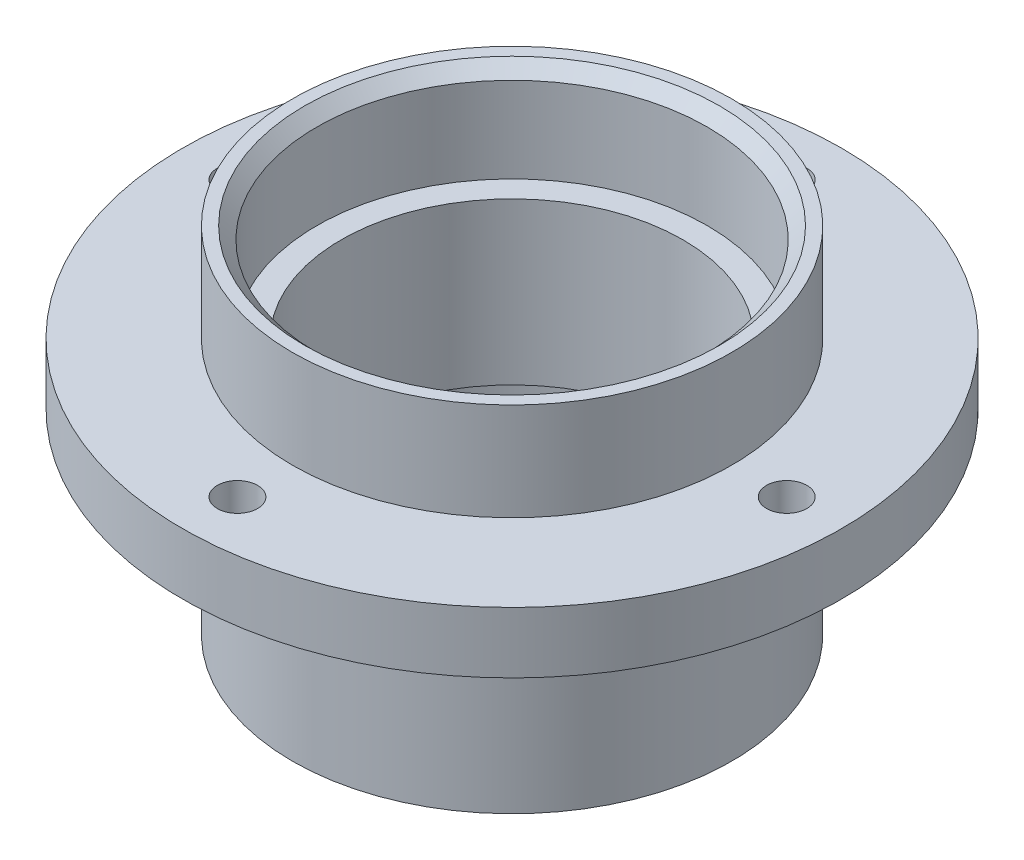
from build123d import *

# Parameters (mm, degrees)
SKETCH1_R             = 18
BOSS_EXTRUDE1_DEPTH   = 8
CUT_EXTRUDE1_REACH    = 28.683
SKETCH2_R             = 16
SKETCH3_R             = 27
BOSS_EXTRUDE2_DEPTH   = 5
BOSS_EXTRUDE3_START   = 16
SKETCH4_R             = 18
BOSS_EXTRUDE3_DEPTH   = 16
SKETCH5_R             = 16
CUT_EXTRUDE2_DEPTH    = 7.8
SKETCH6_R             = 14
CUT_EXTRUDE3_DEPTH    = 44.577517139
M4_TAPPED_HOLE1_D     = 3.3
M4_TAPPED_HOLE1_DEPTH = 11.5
M4_TAPPED_HOLE1_TIP   = 0.991420021
CHAMFER1_SIZE         = 1


with BuildPart() as part:
    # Sketch1 → Boss-Extrude1 (new body)
    with BuildSketch(Plane(origin=(0, 0, 0), x_dir=(1, 0, 0), z_dir=(0, 1, 0))):
        with Locations(Location((0, 0, 0), (0, 0, 270))):
            Circle(SKETCH1_R)
    extrude(amount=BOSS_EXTRUDE1_DEPTH)

    # Sketch2 → Cut-Extrude1 (cut, up to next)
    with BuildSketch(Plane.XZ, mode=Mode.PRIVATE) as cut_extrude1_sk1:
        with Locations(Location((0, 0, 0), (0, 0, 270))):
            Circle(SKETCH2_R)
    cut_extrude1_tool1 = extrude(cut_extrude1_sk1.sketch, amount=-CUT_EXTRUDE1_REACH, mode=Mode.PRIVATE) & part.part
    add(cut_extrude1_tool1.solids().sort_by_distance((0, 0, 0))[0], mode=Mode.SUBTRACT)

    # Sketch3 → Boss-Extrude2 (add)
    with BuildSketch(Plane.XZ):
        with Locations(Location((0, 0, 0), (0, 0, 270))):
            Circle(SKETCH3_R)
    extrude(amount=BOSS_EXTRUDE2_DEPTH)

    # Sketch4 → Boss-Extrude3 (add)
    with BuildSketch(Plane.XZ.offset(5).offset(BOSS_EXTRUDE3_START)):
        with Locations(Location((0, 0, 0), (0, 0, 270))):
            Circle(SKETCH4_R)
    extrude(amount=-BOSS_EXTRUDE3_DEPTH)

    # Sketch5 → Cut-Extrude2 (cut)
    with BuildSketch(Plane.XZ.offset(21)):
        with Locations(Location((0, 0, 0), (0, 0, 270))):
            Circle(SKETCH5_R)
    extrude(amount=-CUT_EXTRUDE2_DEPTH, mode=Mode.SUBTRACT)

    # Sketch6 → Cut-Extrude3 (cut, through all)
    with BuildSketch(Plane(origin=(0, 0, 0), x_dir=(1, 0, 0), z_dir=(0, 1, 0))):
        with Locations(Location((0, 0, 0), (0, 0, 270))):
            Circle(SKETCH6_R)
    extrude(amount=-CUT_EXTRUDE3_DEPTH, mode=Mode.SUBTRACT)

    # M4 Tapped Hole1
    with Locations(Plane(origin=(0, 0, 0), x_dir=(1, 0, 0), z_dir=(0, 1, 0))):
        with Locations((-22.5, 0), (0, 0), (0, 22.5), (22.5, 0), (0, -22.5)):
            Hole(M4_TAPPED_HOLE1_D / 2, depth=M4_TAPPED_HOLE1_DEPTH)
            with Locations((0, 0, -(M4_TAPPED_HOLE1_DEPTH + M4_TAPPED_HOLE1_TIP / 2))):  # 118° drill point
                Cone(0, M4_TAPPED_HOLE1_D / 2, M4_TAPPED_HOLE1_TIP, mode=Mode.SUBTRACT)

    # Chamfer1
    chamfer1_edges = [part.edges().sort_by_distance(p)[0] for p in [
        (0, -21, 16),
        (0, 8, 16),
    ]]
    chamfer(chamfer1_edges, length=CHAMFER1_SIZE)


solid = part.part
